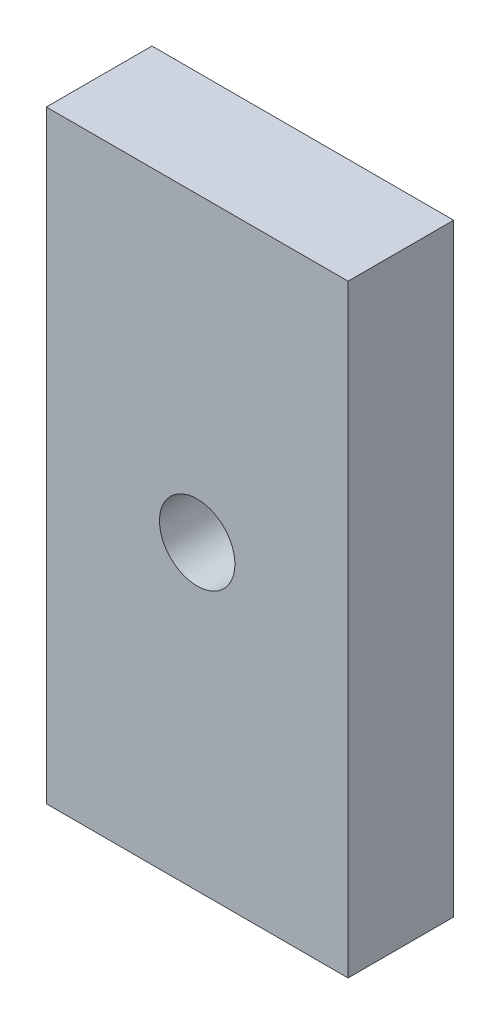
SolidWorks part; units mm, degrees
material "Q235"
ref_plane "Front Plane" through (0, 0, 0) normal (0, 0, 1) x (1, 0, 0)
ref_plane "Top Plane" through (0, 0, 0) normal (0, 1, 0) x (1, 0, 0)
ref_plane "Right Plane" through (0, 0, 0) normal (1, 0, 0) x (0, 0, -1)
sketch "Sketch1" plane through (0, 0, 0) normal (0, 0, 1) x (1, 0, 0)
  line L0 (0, 0) -> (40, 0)
  line L1 (40, 0) -> (40, 80)
  line L2 (40, 80) -> (0, 80)
  line L3 (0, 80) -> (0, 0)
  circle A0 centre (20, 40) radius 5
  dimension "D3" = 10
  dimension "D1" = 40
  dimension "D2" = 80
  dimension "D4" = 40
  dimension "D5" = 20
extrude "Boss-Extrude1" add sketch "Sketch1" along normal blind 14
hole_wizard "M20 Tapped Hole3" positions "Sketch6" profile "Sketch7" tap size "M20" standard "GB"
sketch "Sketch6" plane through (0, 0, 0) normal (0, 0, -1) x (-1, 0, 0)
  point P0 (-20, 40)
sketch "Sketch7" plane through (20, 40, 0) normal (1, 0, 0) x (0, 1, 0)
  line L0 (0, 0) -> (0, 14)
  line L1 (0, 14) -> (8.75, 14)
  line L2 (8.75, 14) -> (8.75, 0)
  line L5 (8.75, 0) -> (0, 0)
  line L11 (0, -6.35) -> (0, 107.95) construction
  dimension "通孔螺纹孔钻头直径" = 17.5
  dimension "通孔螺纹孔钻头深度" = 14
cosmetic thread "Hole thread1" [suppressed] parameters "D2"=20
